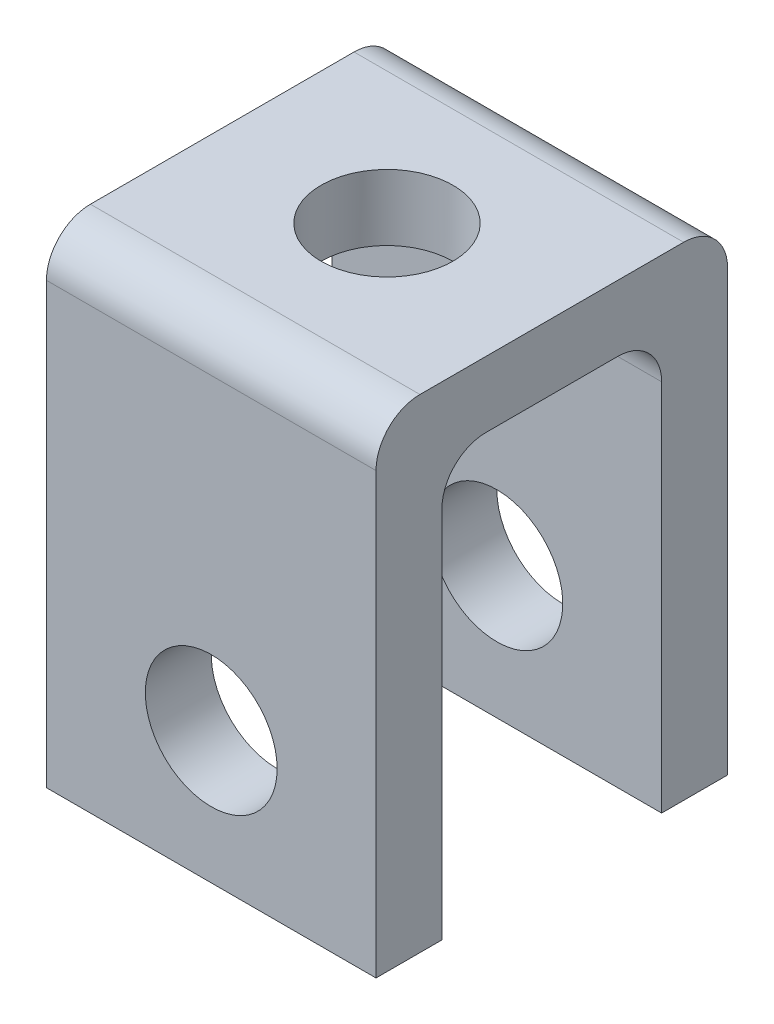
SolidWorks part; units mm, degrees
ref_plane "Front Plane" through (0, 0, 0) normal (0, 0, 1) x (1, 0, 0)
ref_plane "Top Plane" through (0, 0, 0) normal (0, 1, 0) x (1, 0, 0)
ref_plane "Right Plane" through (0, 0, 0) normal (1, 0, 0) x (0, 0, -1)
sketch "Sketch1" plane through (0, 0, 0) normal (0, 0, 1) x (1, 0, 0)
  line L1 (-7.5, -6) -> (7.5, -6)
  line L2 (-7.5, -6) -> (-7.5, 16)
  line L3 (-7.5, 16) -> (7.5, 16)
  line L4 (7.5, -6) -> (7.5, 16)
  circle A0 centre (0, 0) radius 3
  dimension "D1" = 6
  dimension "D5" = 6
  dimension "D2" = 15
  dimension "D3" = 7.5
  dimension "D4" = 22
extrude "Boss-Extrude1" add sketch "Sketch1" along normal mid plane 16
sketch "Sketch2" plane through (7.5, 0, 0) normal (1, 0, 0) x (0, 0, -1)
  line L0 (-8, -6) -> (8, -6) construction
  line L1 (-5, -6) -> (5, -6)
  line L2 (-5, -6) -> (-5, 13)
  line L3 (-5, 13) -> (5, 13)
  line L4 (5, -6) -> (5, 13)
  line L5 (-8, 16) -> (8, 16) construction
  dimension "D1" = 10
  dimension "D2" = 5
  dimension "D3" = 3
extrude "Cut-Extrude1" cut sketch "Sketch2" against normal through all
fillet "Fillet1" radius 2 4 edges at (0, 13, -5) (0, 16, -8) (0, 16, 8) (0, 13, 5)
sketch "Sketch3" plane through (0, 16, 0) normal (0, 1, 0) x (1, 0, 0)
  circle A0 centre (0, 0) radius 3
  dimension "D1" = 6
extrude "Cut-Extrude2" cut sketch "Sketch3" against normal blind 18
